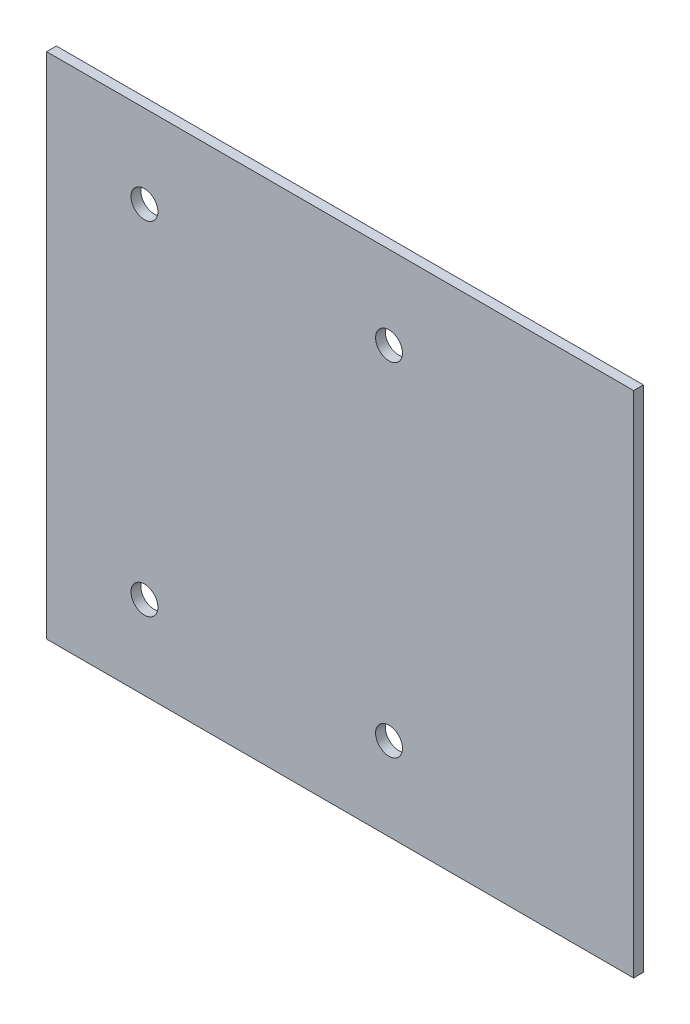
from build123d import *

# Parameters (mm, degrees)
SKETCH_1_W          = 240
SKETCH_1_H          = 208
EXTRUDE_1_DEPTH     = 4
SKETCH_2_R          = 5.5
CUT_EXTRUDE_1_DEPTH = 10


with BuildPart() as part:
    # 草图1 → 凸台-拉伸1 (new body)
    with BuildSketch(Plane.XY):
        Rectangle(SKETCH_1_W, SKETCH_1_H)
    extrude(amount=EXTRUDE_1_DEPTH)

    # 草图2 → 切除-拉伸1 (cut)
    with BuildSketch(Plane(origin=(0, 0, 0), x_dir=(-1, 0, 0), z_dir=(0, 0, -1))):
        with Locations((-20, -70)):
            Circle(SKETCH_2_R)
        with Locations((80, -70)):
            Circle(SKETCH_2_R)
        with Locations((80, 70)):
            Circle(SKETCH_2_R)
        with Locations((-20, 70)):
            Circle(SKETCH_2_R)
    extrude(amount=-CUT_EXTRUDE_1_DEPTH, mode=Mode.SUBTRACT)


solid = part.part
